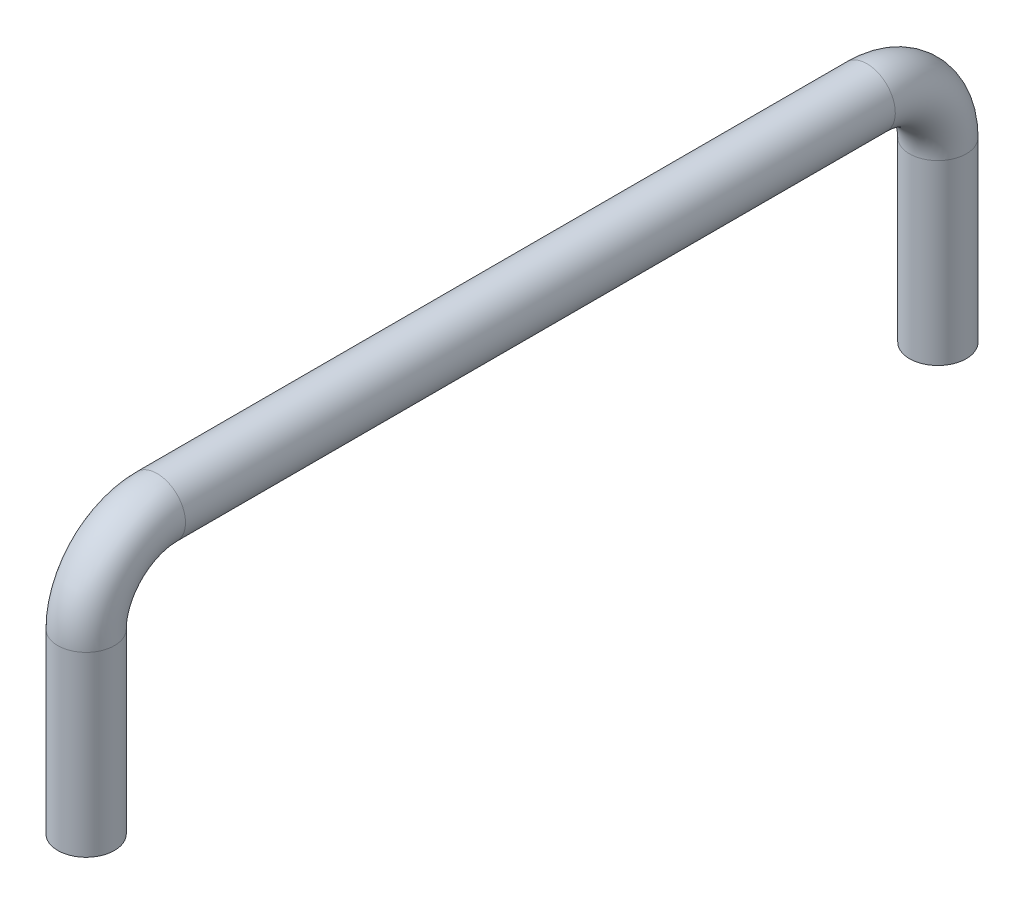
SolidWorks part; units mm, degrees
ref_plane "Front Plane" through (0, 0, 0) normal (0, 0, 1) x (1, 0, 0)
ref_plane "Top Plane" through (0, 0, 0) normal (0, 1, 0) x (1, 0, 0)
ref_plane "Right Plane" through (0, 0, 0) normal (1, 0, 0) x (0, 0, -1)
sketch "Sketch1" plane through (0, 0, 0) normal (1, 0, 0) x (0, 0, -1)
  line L0 (-76.2, 101.6) -> (76.2, 101.6) construction
  line L1 (-76.2, 57.15) -> (-76.2, 101.6) construction
  line L2 (76.2, 101.6) -> (76.2, 57.15) construction
  line L3 (-63.5, 101.6) -> (63.5, 101.6)
  line L4 (-76.2, 57.15) -> (-76.2, 88.9)
  line L5 (76.2, 88.9) -> (76.2, 57.15)
  arc A0 (63.5, 101.6) -> (76.2, 88.9) centre (63.5, 88.9) cw
  arc A1 (-63.5, 101.6) -> (-76.2, 88.9) centre (-63.5, 88.9) ccw
  dimension "D1" = 12.7
ref_plane "Plane1" through (0, 57.15, 76.2) normal (0, 1, 0) x (-1, 0, 0)
sketch "Sketch2" plane through (0, 57.15, 76.2) normal (0, 1, 0) x (-1, 0, 0)
  circle A0 centre (0, 0) radius 5.08
  dimension "D1" = 10.16
sweep "Sweep1" add profiles "Sketch2" path "Sketch1"
